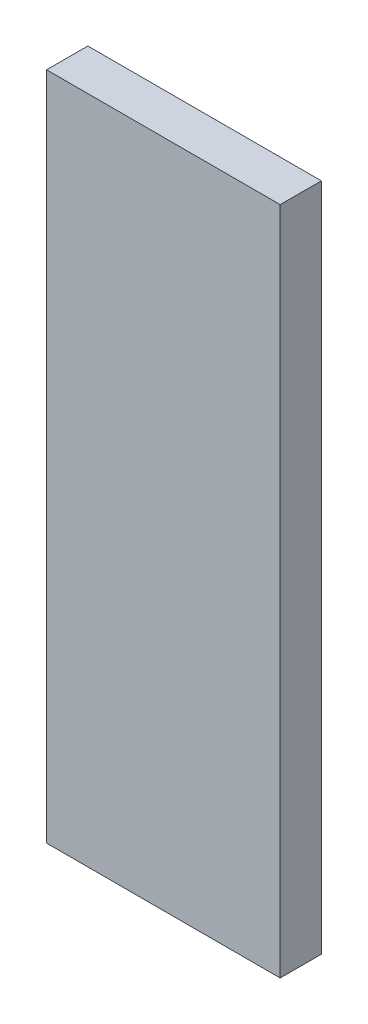
SolidWorks part; units mm, degrees
ref_plane "Front Plane" through (0, 0, 0) normal (0, 0, 1) x (1, 0, 0)
ref_plane "Top Plane" through (0, 0, 0) normal (0, 1, 0) x (1, 0, 0)
ref_plane "Right Plane" through (0, 0, 0) normal (1, 0, 0) x (0, 0, -1)
sketch "Sketch1" plane through (0, 0, 0) normal (0, 0, 1) x (1, 0, 0)
  line L1 (0, 0) -> (68, 0)
  line L2 (0, 0) -> (0, 195)
  line L3 (0, 195) -> (68, 195)
  line L4 (68, 0) -> (68, 195)
  dimension "D1" = 195
  dimension "D2" = 68
extrude "Boss-Extrude1" add sketch "Sketch1" along normal blind 12
